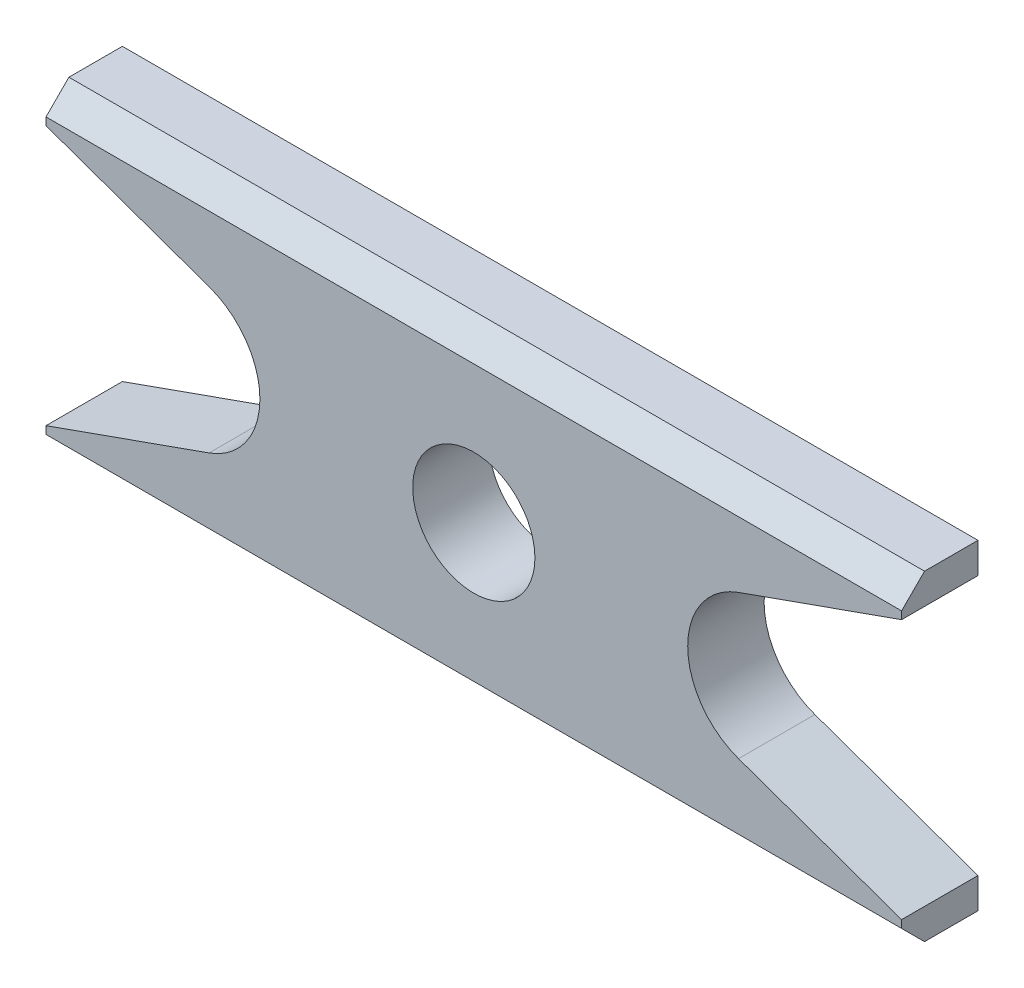
from build123d import *

# Parameters (mm, degrees)
SKETCH1_R           = 40
BOSS_EXTRUDE1_DEPTH = 25
CHAMFER1_SIZE       = 15


with BuildPart() as part:
    # Sketch1 → Boss-Extrude1 (new, symmetric)
    with BuildSketch(Plane.XY):
        with BuildLine():
            Line((-280, 105), (280, 105))
            Line((280, 105), (280, 85))
            Line((280, 85), (173.275566379, 47.11998854))
            ThreePointArc((173.275566379, 47.11998854), (140, 0), (173.275566379, -47.11998854))
            Line((173.275566379, -47.11998854), (280, -85))
            Line((280, -85), (280, -105))
            Line((280, -105), (-280, -105))
            Line((-280, -105), (-280, -85))
            Line((-280, -85), (-173.275566379, -47.11998854))
            ThreePointArc((-173.275566379, -47.11998854), (-140, 0), (-173.275566379, 47.11998854))
            Line((-173.275566379, 47.11998854), (-280, 85))
            Line((-280, 85), (-280, 105))
        make_face()
        Circle(SKETCH1_R, mode=Mode.SUBTRACT)
    extrude(amount=BOSS_EXTRUDE1_DEPTH, both=True)

    # Chamfer1
    chamfer1_edges = [part.edges().sort_by_distance(p)[0] for p in [
        (0, 105, 25),
        (0, -105, 25),
    ]]
    chamfer(chamfer1_edges, length=CHAMFER1_SIZE)


solid = part.part
